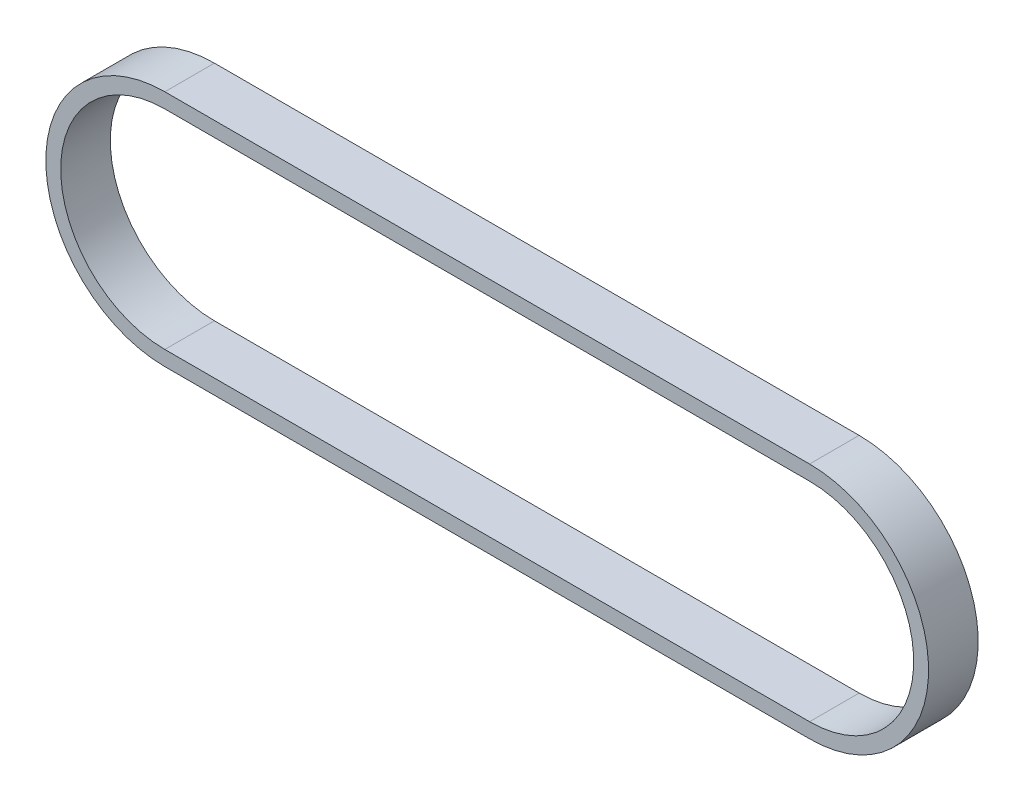
SolidWorks part; units mm, degrees
ref_plane "Front Plane" through (0, 0, 0) normal (0, 0, 1) x (1, 0, 0)
ref_plane "Top Plane" through (0, 0, 0) normal (0, 1, 0) x (1, 0, 0)
ref_plane "Right Plane" through (0, 0, 0) normal (1, 0, 0) x (0, 0, -1)
sketch "Sketch2" plane through (0, 0, 0) normal (0, 0, 1) x (1, 0, 0)
  line L0 (5.5, 0) -> (-5.5, 0) construction
  line L1 (0, 24) -> (-130, 24)
  line L2 (0, -24) -> (-130, -24)
  arc A0 (0, -24) -> (0, 24) centre (0, 0) ccw
  arc A1 (-130, 24) -> (-130, -24) centre (-130, 0) ccw
  dimension "D1" = 48
  dimension "D2" = 48
  dimension "D3" = 130
extrude "Boss-Extrude1" add sketch "Sketch2" along normal blind 10
shell "Shell1" thickness 3
